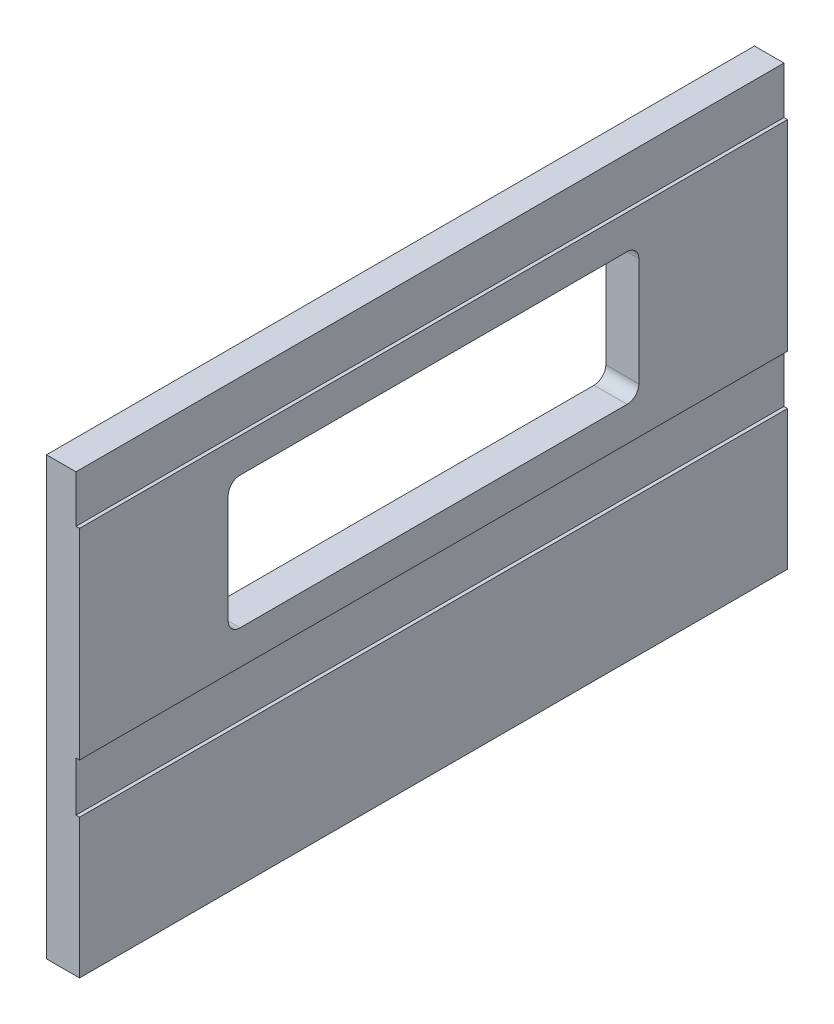
SolidWorks part; units mm, degrees
ref_plane "前视基准面" through (0, 0, 0) normal (0, 0, 1) x (1, 0, 0)
ref_plane "上视基准面" through (0, 0, 0) normal (0, 1, 0) x (1, 0, 0)
ref_plane "右视基准面" through (0, 0, 0) normal (1, 0, 0) x (0, 0, -1)
sketch "草图1" plane through (0, 0, 0) normal (0, 0, 1) x (1, 0, 0)
  line L0 (0, 0) -> (0, 185)
  line L1 (0, 185) -> (14, 185)
  line L2 (14, 185) -> (14, 0)
  line L6 (0, 0) -> (14, 0)
  dimension "D2" = 14
  dimension "D4" = 185
extrude "凸台-拉伸1" add sketch "草图1" along normal mid plane 300
sketch "草图2" plane through (14, 0, 0) normal (1, 0, 0) x (0, 0, -1)
  line L0 (150, 0) -> (150, 185) construction
  line L1 (-150, 185) -> (150, 185)
  line L2 (-150, 185) -> (-150, 165)
  line L3 (-150, 165) -> (150, 165)
  line L4 (150, 185) -> (150, 165)
  line L5 (-150, 0) -> (-150, 185) construction
  line L6 (-150, 80) -> (150, 80)
  line L7 (-150, 80) -> (-150, 59)
  line L8 (-150, 59) -> (150, 59)
  line L9 (150, 80) -> (150, 59)
  dimension "D1" = 20
  dimension "D2" = 21
  dimension "D3" = 85
extrude "切除-拉伸1" cut sketch "草图2" against normal blind 1.5
sketch "草图3" plane through (14, 0, 0) normal (1, 0, 0) x (0, 0, -1)
  line L0 (0, 122.5) -> (150, 122.5) construction
  line L1 (-87, 94.5) -> (87, 94.5)
  line L2 (-87, 94.5) -> (-87, 150.5)
  line L3 (-87, 150.5) -> (87, 150.5)
  line L4 (87, 94.5) -> (87, 150.5)
  line L5 (-87, 94.5) -> (87, 150.5) construction
  line L6 (-87, 150.5) -> (87, 94.5) construction
  line L7 (150, 80) -> (150, 165) construction
  point P0 (0, 122.5)
  dimension "D1" = 56
  dimension "D2" = 174
extrude "切除-拉伸2" cut sketch "草图3" against normal up to next
fillet "圆角1" radius 5 4 edges at (7, 94.5, 87) (7, 150.5, 87) (7, 94.5, -87) (7, 150.5, -87)
sketch "草图4" plane through (0, 0, 150) normal (0, 0, 1) x (1, 0, 0)
  line L0 (0, 185) -> (0, 0) construction
  line L1 (0, 77) -> (14, 77)
  line L2 (0, 77) -> (0, 65)
  line L3 (0, 65) -> (14, 65)
  line L4 (14, 77) -> (14, 65)
  line L5 (14, 80) -> (14, 165) construction
  line L6 (0, 0) -> (14, 0) construction
  dimension "D1" = 12
  dimension "D2" = 65
extrude "凸台-拉伸2" [suppressed] add sketch "草图4" along normal blind 12
